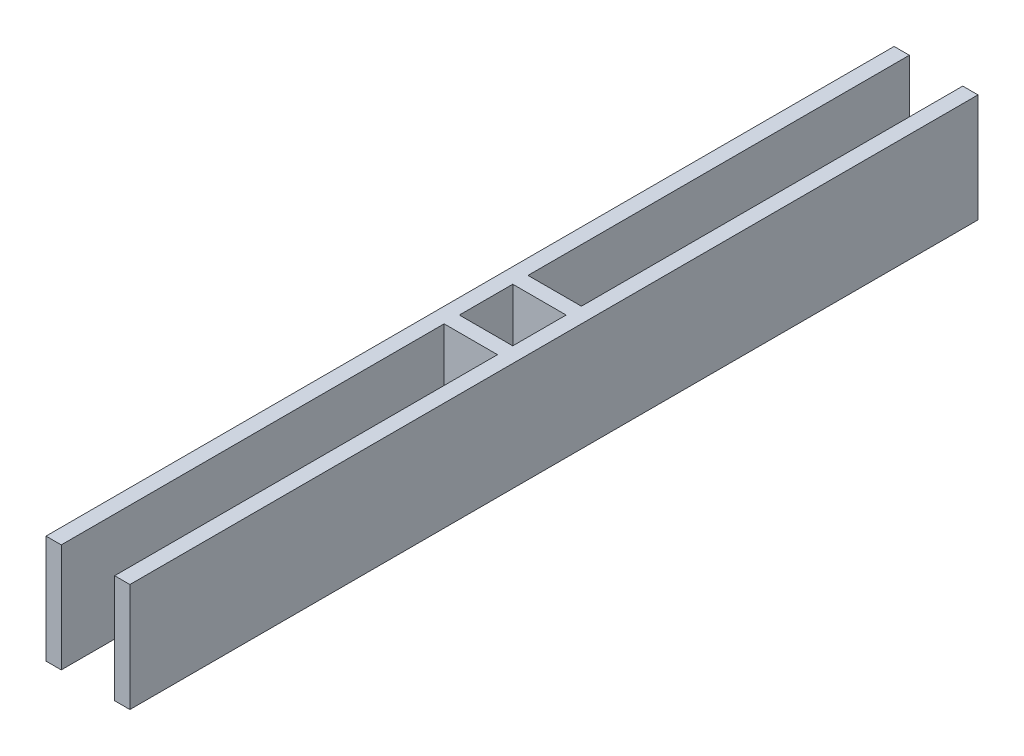
SolidWorks part; units mm, degrees
ref_plane "Front Plane" through (0, 0, 0) normal (0, 0, 1) x (1, 0, 0)
ref_plane "Top Plane" through (0, 0, 0) normal (0, 1, 0) x (1, 0, 0)
ref_plane "Right Plane" through (0, 0, 0) normal (1, 0, 0) x (0, 0, -1)
other "Configuration Table"
sketch "Sketch1" plane through (0, 0, 0) normal (0, 0, 1) x (1, 0, 0)
  line L1 (-5, 35.5) -> (5, 35.5)
  line L2 (-5, 35.5) -> (-5, -35.5)
  line L3 (-5, -35.5) -> (5, -35.5)
  line L4 (5, 35.5) -> (5, -35.5)
  line L5 (-5, 35.5) -> (5, -35.5) construction
  line L6 (-5, -35.5) -> (5, 35.5) construction
  point P0 (0, 0)
  dimension "D1" = 10
  dimension "D2" = 71
extrude "Boss-Extrude1" add sketch "Sketch1" along normal blind 556
sketch "Sketch2" plane through (5, 0, 0) normal (1, 0, 0) x (0, 0, -1)
  line L0 (-556, -35.5) -> (0, -35.5) construction
  line L1 (-305, 35.5) -> (-295, 35.5)
  line L2 (-305, 35.5) -> (-305, -35.5)
  line L3 (-305, -35.5) -> (-295, -35.5)
  line L4 (-295, 35.5) -> (-295, -35.5)
  line L5 (-305, 35.5) -> (-295, -35.5) construction
  line L6 (-305, -35.5) -> (-295, 35.5) construction
  line L7 (0, -35.5) -> (0, 35.5) construction
  line L8 (-260, 35.5) -> (-250, 35.5)
  line L9 (-260, 35.5) -> (-260, -35.5)
  line L10 (-260, -35.5) -> (-250, -35.5)
  line L11 (-250, 35.5) -> (-250, -35.5)
  line L12 (-260, 35.5) -> (-250, -35.5) construction
  line L13 (-260, -35.5) -> (-250, 35.5) construction
  point P0 (-300, 0)
  point P7 (-255, 0)
  dimension "D1" = 10
  dimension "D2" = 10
  dimension "D3" = 55
  dimension "D4" = 250
extrude "Boss-Extrude2" add sketch "Sketch2" along normal blind 35
sketch "Sketch3" plane through (0, 35.5, 0) normal (0, 1, 0) x (1, 0, 0)
  line L1 (40, -556) -> (50, -556)
  line L2 (40, -556) -> (40, 0)
  line L3 (40, 0) -> (50, 0)
  line L4 (50, -556) -> (50, 0)
  dimension "D1" = 10
extrude "Boss-Extrude3" add sketch "Sketch3" against normal blind 71
